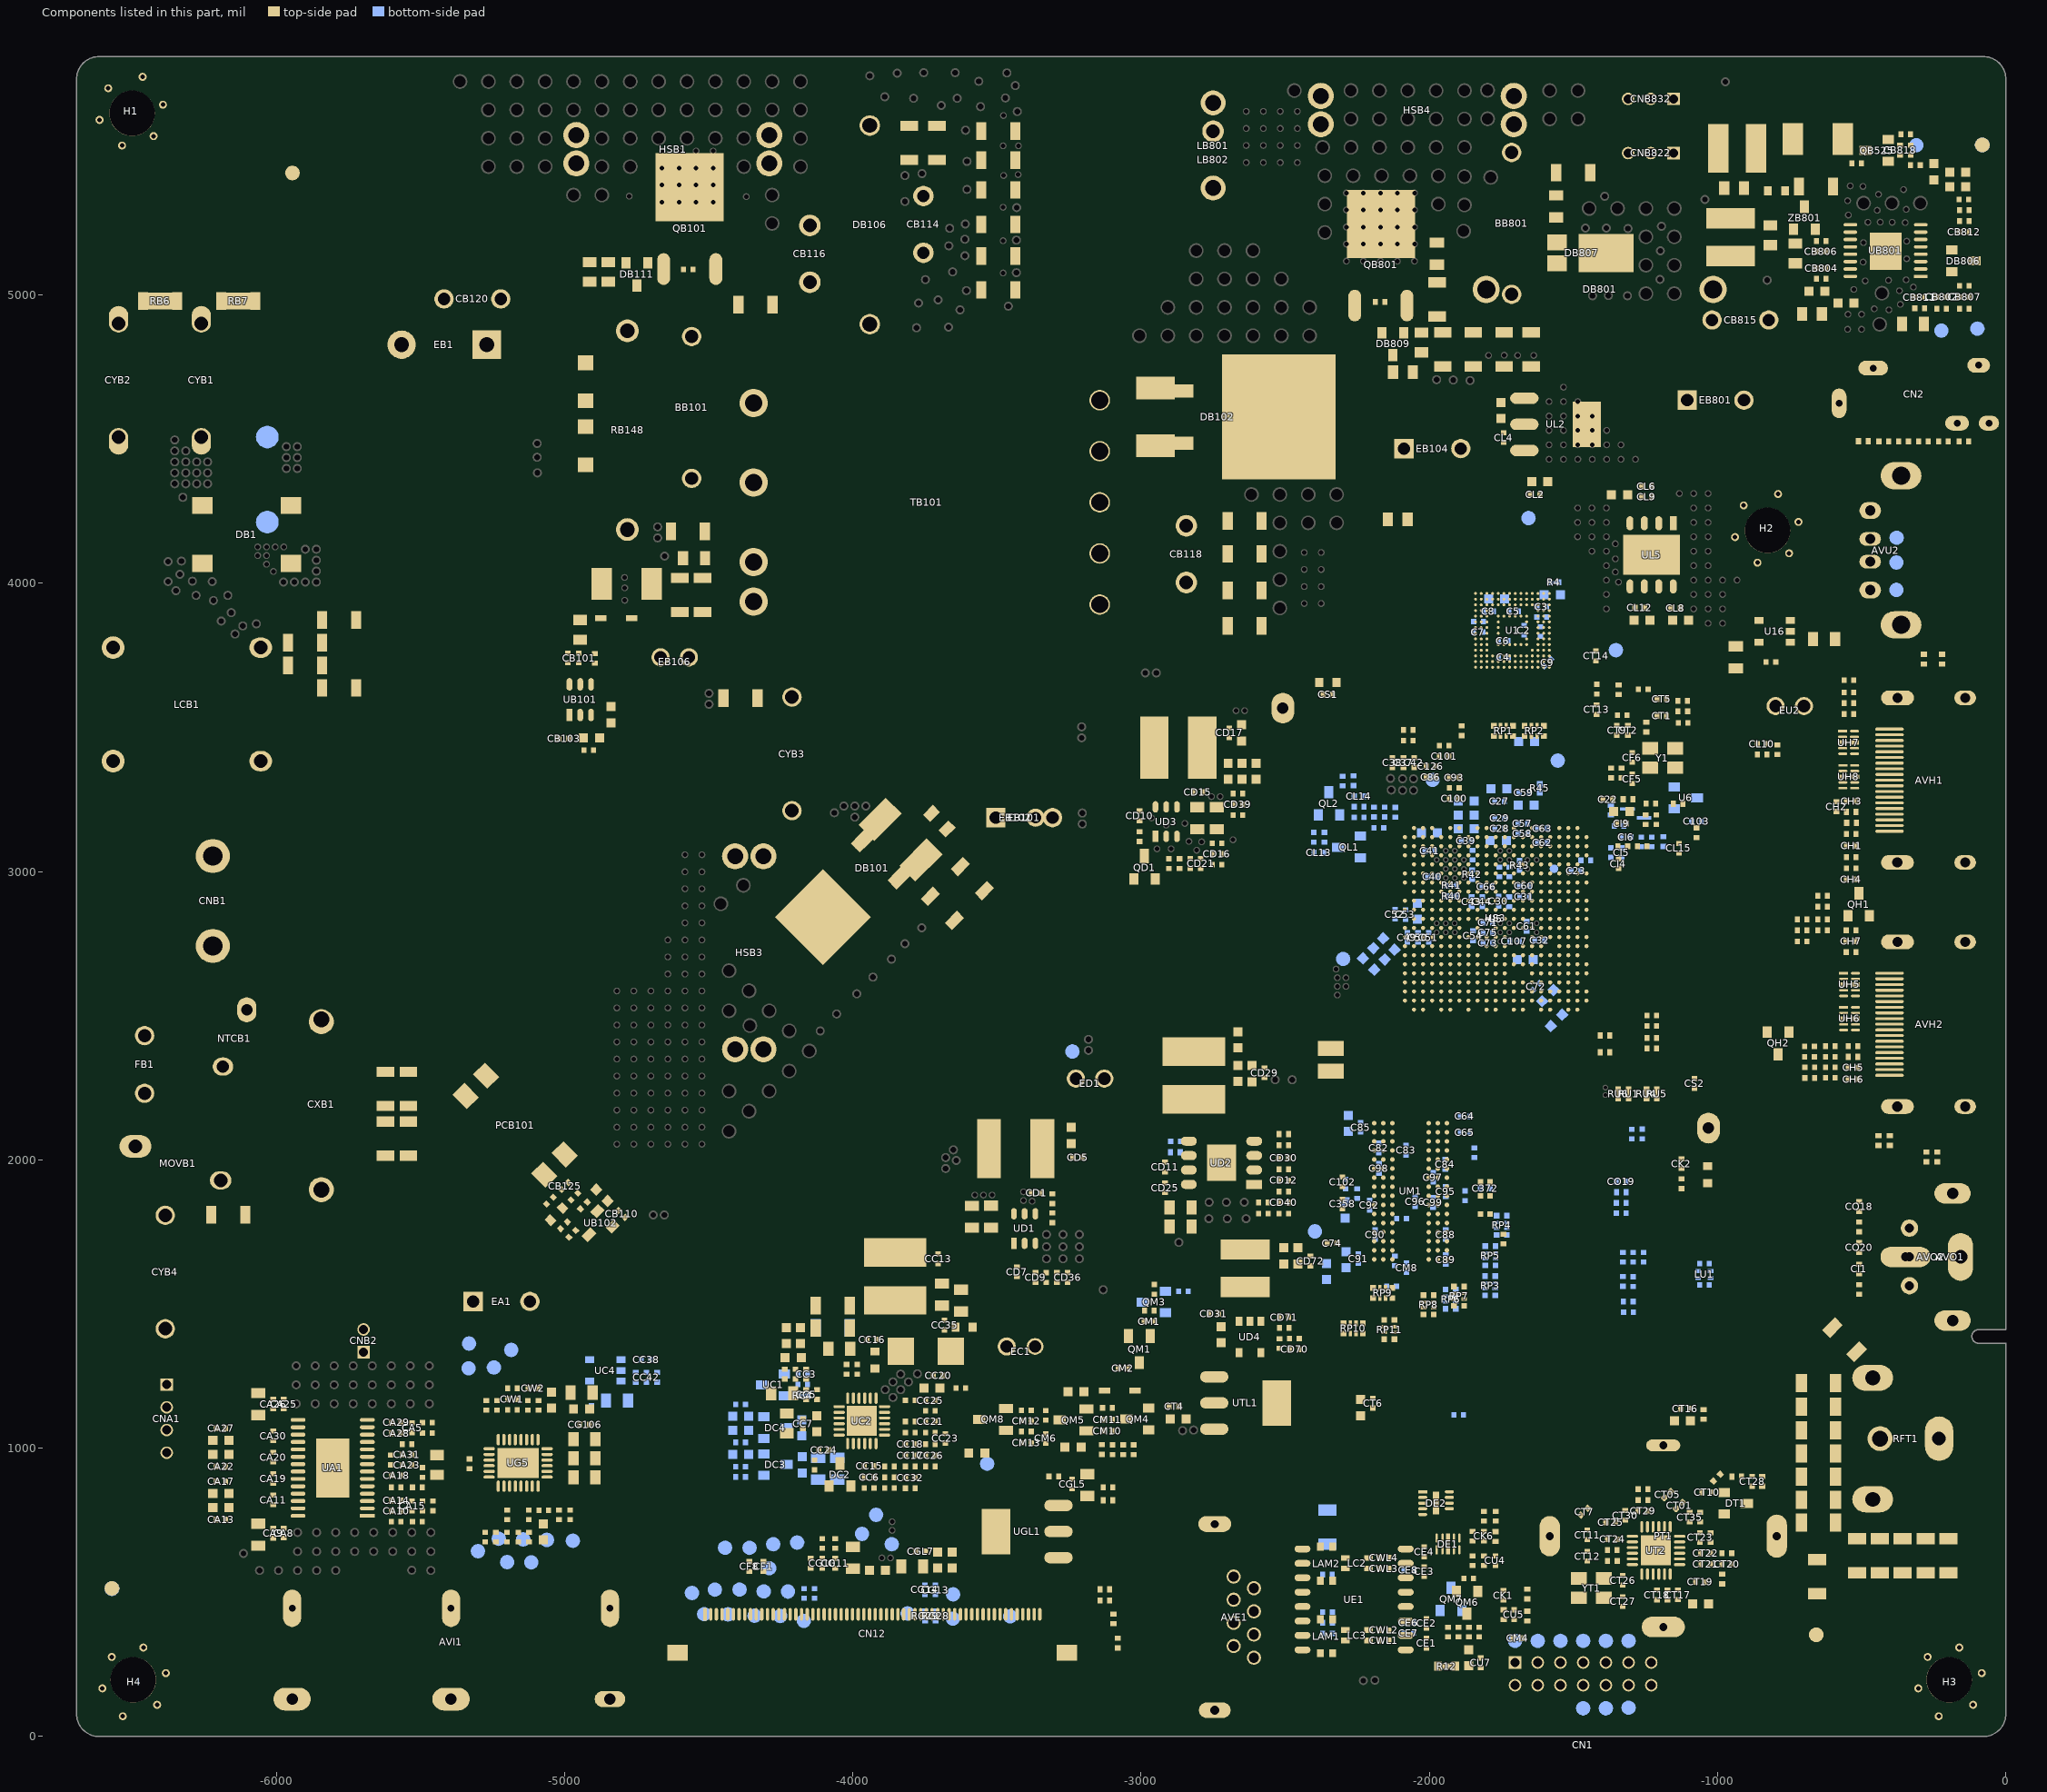
[diagram p0: the components of this part, seen from the top]
# Altium PCB MISC84395.PcbDoc (part 26 of 26)
Units mil, origin at the board's own origin, x right, y up, seen from the top; angles counter-clockwise.
Board outline 6692.91 x 5826.77 mil, 2 copper layers (TopLayer, BottomLayer), stack 61.855 mil thick; 951 components, 565 nets, 4374 pads, 1804 vias.
Unrouted connection lines stored in the file: 1.

## Silkscreen, mask and mechanical layers (free items; w line width, h text height) (continued)
附加说明:
  lines w5: -6671,5609.76 -78.74,5610.24 ; -157.48,-66 -157.48,5855 ; 7256.74,4932.99 8386.74,4932.99 ; 7256.74,5040.32 8386.74,5040.32 ; 7256.74,5147.65 8386.74,5147.65 ; 7256.74,5254.99 8386.74,5254.99 ; 7256.74,5362.32 8687.24,5362.32 ; 7557.24,4825.65 7557.24,5469.65 ; 8386.74,4825.65 8386.74,5469.65 ; 7256.74,4825.65 8687.24,4825.65 8687.24,5469.65 7256.74,5469.65 7256.74,4825.65
  text "Template date:" at 5060.58,5397.67 h60
  text "Version/cycle number" at 7278.58,5396.5 h60
  text "PCB designer" at 7834.08,5396 h60
  text "Customer" at 8497.08,5396.5 h60
  text "2018.12.27" at 5382.58,5394.17 h60
  text "Board utilisation:" at 5060.08,5300.67 h60
  text "8X%" at 5382.58,5296.67 h60
  text "(Fill in for non-TV business unit projects)" at 5572.58,5296.67 h60
  text "XXXXXX" at 7298.08,5289.5 h60
  text "HYW  PXK   WW" at 7602.08,5288.67 h60
  text "ZFB" at 7621,5193 h60
  text "XXXXXX" at 7294.08,5191.5 h60
  text "COMPANY_A" at 8426.08,5079.17 h60
  text "LCF" at 7619.5,5075 h60
  text "XXXXXX" at 7292.58,5073.5 h60
  text "XXXXXX" at 7296.08,4970.5 h60
  text "ZFB" at 7620.5,4964 h60
  text "Special requirements; leave blank if none" at 3650.74,4900.01 h60
  text "The remark items below must be copied to the TopOverlay layer; one or two items may be remarked" at 4648.08,2319.17 h60
  text "Only one barcode position on board; the other barcode must be attached to the component" at 6166.71,2316.27 h60
  text "No barcode position on board; barcode must be attached to the component" at 6166.71,2237.07 h60
  text "Height values and designators of SMD components above 2mm on the solder side; leave blank if none" at 3941.13,2024.21 h60
  text "Designators of components prone to collision; leave blank if none" at 3939.36,1878.05 h60
  text "Suction cup and press bar positions reserved: enter 'Yes'; otherwise enter 'No'" at 3942.58,1468.17 h60
  text "X.XXXX.XXX Stencil Revision Explanation" at 3015.36,-1351.8 h60
  text "X.XXXX.XXX Testing jig Revision Explanation" at 3014.86,-1420.8 h60
  text "X.XXXX.XXX Wave-soldering jig Revision Explanation" at 3014.36,-1488.8 h60
DrillDrawing:
  text ".Legend" at 3023.4,5517.89 h60